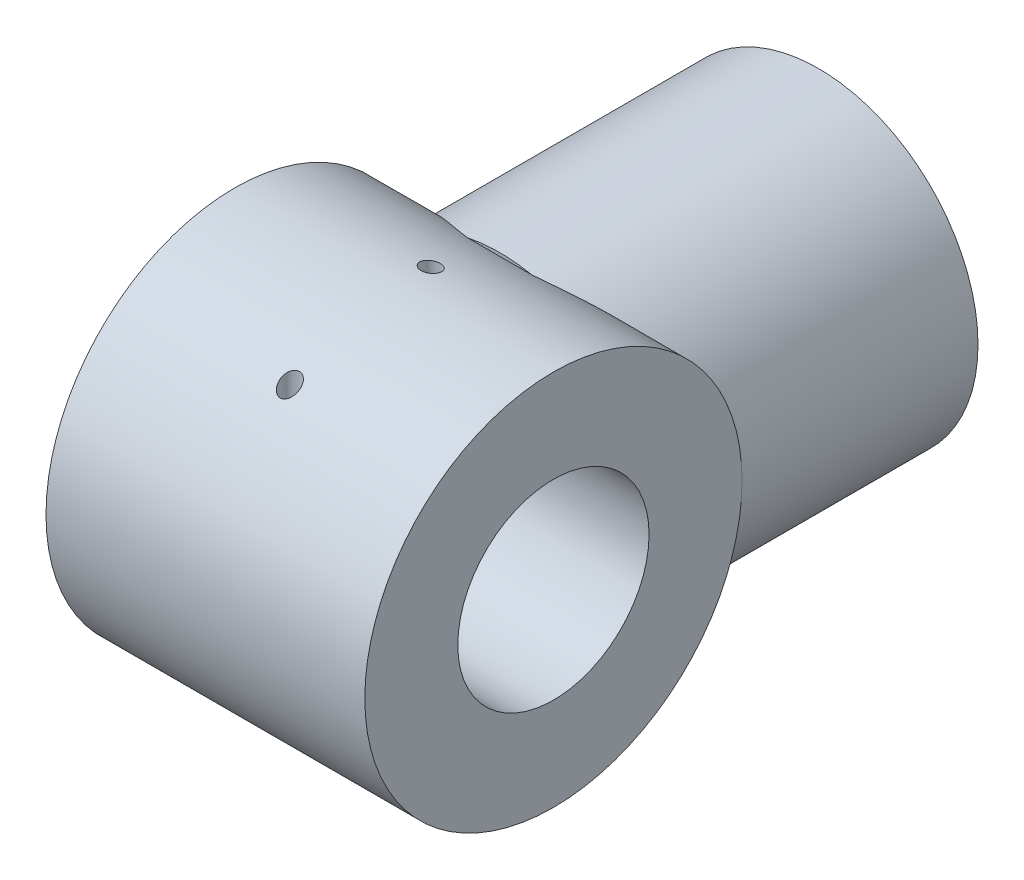
from build123d import *

# Parameters (mm, degrees)
SKETCH1_R           = 25
BOSS_EXTRUDE1_DEPTH = 50
SKETCH3_R           = 29.577748383
BOSS_EXTRUDE2_DEPTH = 25
SKETCH4_R           = 15
BOSS_EXTRUDE3_DEPTH = 5
CUT_EXTRUDE1_REACH  = 118.762
SKETCH5_R           = 15
SKETCH6_R           = 1.5
CUT_EXTRUDE2_DEPTH  = 20


with BuildPart() as part:
    # Sketch1 → Boss-Extrude1 (new body)
    with BuildSketch(Plane.XY):
        with Locations((-138.044677266, -13.853162466)):
            Circle(SKETCH1_R)
    extrude(amount=BOSS_EXTRUDE1_DEPTH)

    # Sketch3 → Boss-Extrude2 (add, symmetric)
    with BuildSketch(Plane(origin=(-138.044677266, 0, 0), x_dir=(0, 0, -1), z_dir=(1, 0, 0))):
        with Locations((-66.584372838, -13.853162466)):
            Circle(SKETCH3_R)
    extrude(amount=BOSS_EXTRUDE2_DEPTH, both=True)

    # Sketch4 → Boss-Extrude3 (add, symmetric)
    with BuildSketch(Plane(origin=(0, 0, 0), x_dir=(-1, 0, 0), z_dir=(0, 0, -1))):
        with Locations(Location((138.044677266, -13.853162466, 0), (0, 0, 180))):
            Circle(SKETCH4_R)
    extrude(amount=BOSS_EXTRUDE3_DEPTH, both=True)

    # Sketch5 → Cut-Extrude1 (cut, up to next)
    with BuildSketch(Plane.ZY.offset(163.044677266), mode=Mode.PRIVATE) as cut_extrude1_sk1:
        with Locations((66.584372838, -13.853162466)):
            Circle(SKETCH5_R)
    cut_extrude1_tool1 = extrude(cut_extrude1_sk1.sketch, amount=-CUT_EXTRUDE1_REACH, mode=Mode.PRIVATE) & part.part
    add(cut_extrude1_tool1.solids().sort_by_distance((-163.044677, -13.853162, 66.584373))[0], mode=Mode.SUBTRACT)

    # Sketch6 → Cut-Extrude2 (cut)
    with BuildSketch(Plane(origin=(0, 0, 0), x_dir=(1, 0, 0), z_dir=(0, 1, 0))):
        with Locations(Location((-137.396937397, -61.478842375, 0), (0, 0, 90))):
            Circle(SKETCH6_R)
        with Locations(Location((-137.396937397, -83.561946624, 0), (0, 0, 90))):
            Circle(SKETCH6_R)
    extrude(amount=CUT_EXTRUDE2_DEPTH, mode=Mode.SUBTRACT)


solid = part.part
